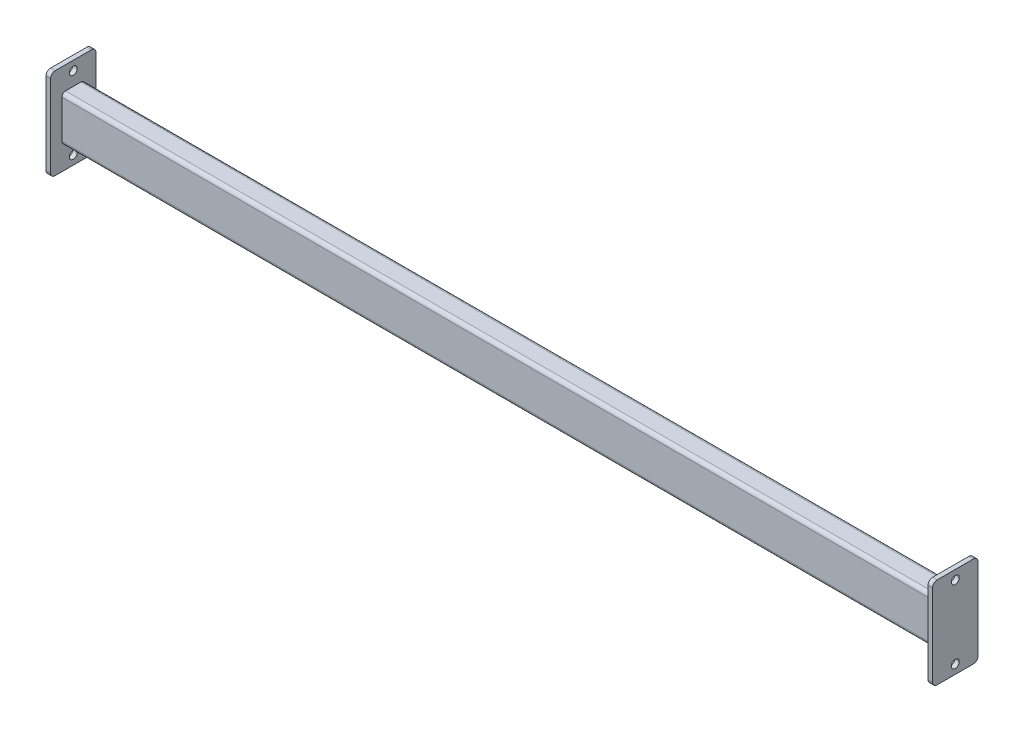
SolidWorks part; units mm, degrees
ref_plane "Front Plane" through (0, 0, 0) normal (0, 0, 1) x (1, 0, 0)
ref_plane "Top Plane" through (0, 0, 0) normal (0, 1, 0) x (1, 0, 0)
ref_plane "Right Plane" through (0, 0, 0) normal (1, 0, 0) x (0, 0, -1)
other "Configuration Table"
sketch "Sketch2" plane through (0, 0, 0) normal (0, 1, 0) x (1, 0, 0)
  line L0 (-965, 0) -> (965, 0)
  point P4 (0, 0)
  dimension "D1" = 1930
other "Gb／6728-1986 rectangular hollow section 100 X 50 X 4 (1)"
ref_plane "Plane1" through (-965, 0, 0) normal (1, 0, 0) x (0, 0, -1)
sketch "Sketch1" plane through (-965, 0, 0) normal (1, 0, 0) x (0, 0, -1)
  line L0 (-17, -46) -> (17, -46)
  line L1 (-21, -42) -> (-21, 42)
  line L2 (17, 46) -> (-17, 46)
  line L3 (21, 42) -> (21, -42)
  line L4 (-17, -50) -> (17, -50)
  line L5 (-25, -42) -> (-25, 42)
  line L6 (17, 50) -> (-17, 50)
  line L7 (25, 42) -> (25, -42)
  arc A0 (25, 42) -> (17, 50) centre (17, 42) ccw
  arc A1 (17, -50) -> (25, -42) centre (17, -42) ccw
  arc A2 (-25, -42) -> (-17, -50) centre (-17, -42) ccw
  arc A3 (-17, 50) -> (-25, 42) centre (-17, 42) ccw
  arc A4 (-17, 46) -> (-21, 42) centre (-17, 42) ccw
  arc A5 (21, 42) -> (17, 46) centre (17, 42) ccw
  arc A6 (17, -46) -> (21, -42) centre (17, -42) ccw
  arc A7 (-21, -42) -> (-17, -46) centre (-17, -42) ccw
  point P0 (0, 50)
  point P1 (25, 0)
  point P2 (0, -50)
  point P3 (-25, 0)
  point P4 (-25, 50)
  point P5 (25, 50)
  point P6 (25, -50)
  point P7 (-25, -50)
  point P8 (0, 0)
  point P33 (0, 0)
  dimension "D1" = 8
  dimension "Thickness" = 4
  dimension "V_leg" = 100
  dimension "H_leg" = 50
sketch "Sketch4" plane through (-965, 0, 0) normal (-1, 0, 0) x (0, 0, 1)
  line L1 (-50, -100) -> (50, -100)
  line L2 (-50, -100) -> (-50, 100)
  line L3 (-50, 100) -> (50, 100)
  line L4 (50, -100) -> (50, 100)
  line L5 (-50, -100) -> (50, 100) construction
  line L6 (-50, 100) -> (50, -100) construction
  point P0 (0, 0)
  dimension "D1" = 100
  dimension "D2" = 200
extrude "Boss-Extrude1" add sketch "Sketch4" along normal blind 10 separate body
ref_plane "Plane2" through (0, 0, 0) normal (-1, 0, 0) x (0, 0, 1)
fillet "Fillet1" radius 10 4 edges at (-970, -100, 50) (-970, -100, -50) (-970, 100, 50) (-970, 100, -50)
mirror "Mirror2" about plane through (0, 0, 0) normal (-1, 0, 0) of bodies 107
hole_wizard "M16 Clearance Hole2" positions "Sketch8" profile "Sketch9" hole size "M16" standard "GB" end condition through all
sketch "Sketch8" plane through (-975, 0, 0) normal (-1, 0, 0) x (0, 0, 1)
  line L0 (0, 100) -> (0, -100) construction
  line L1 (40, 100) -> (-40, 100) construction
  line L2 (-40, -100) -> (40, -100) construction
  line L4 (-50, 0) -> (50, 0) construction
  line L5 (-50, 90) -> (-50, -90) construction
  line L6 (50, -90) -> (50, 90) construction
  point P0 (0, 80)
  point P2 (0, -80)
  dimension "D1" = 160
sketch "Sketch9" plane through (-975, 80, 0) normal (0, 1, 0) x (0, 0, 1)
  line L0 (0, 0) -> (0, 1950)
  line L1 (0, 1950) -> (8.75, 1950)
  line L2 (8.75, 1950) -> (8.75, 0)
  line L5 (8.75, 0) -> (0, 0)
  line L11 (0, -6.35) -> (0, 107.95) construction
  dimension "通孔孔直径" = 17.5
  dimension "通孔孔深度" = 1950
sketch "Sketch10" plane through (965, 0, 0) normal (-1, 0, 0) x (0, 0, 1)
  circle A0 centre (0, -80) radius 12 construction
  dimension "D1" = 24
